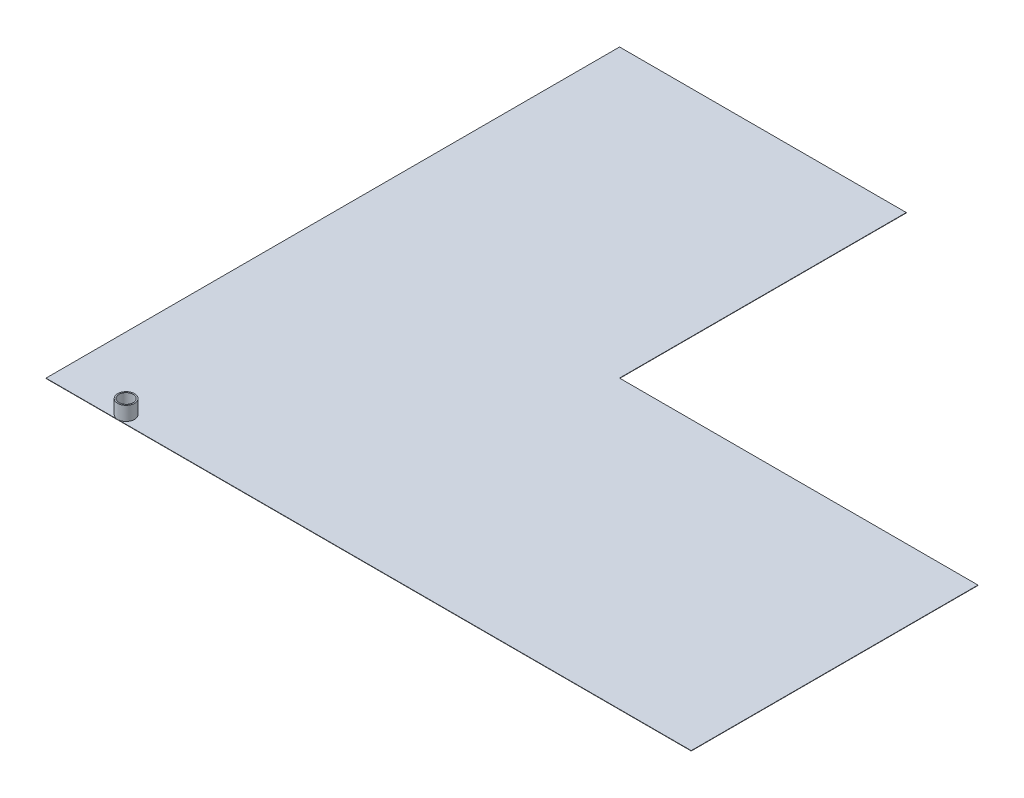
from build123d import *

# Parameters (mm, degrees)
BOSS_EXTRUDE1_DEPTH = 1
SKETCH2_R           = 20
CUT_EXTRUDE1_DEPTH  = 1205.159873107
BOSS_EXTRUDE2_START = 39
SKETCH3_R           = 23.5
SKETCH3_R_2         = 20
BOSS_EXTRUDE2_DEPTH = 39


with BuildPart() as part:
    # Sketch1 → Boss-Extrude1 (new body)
    with BuildSketch(Plane(origin=(0, 0, 0), x_dir=(1, 0, 0), z_dir=(0, 1, 0))):
        Polygon((-900, -800), (900, -800), (900, 0), (0, 0), (-100, 0), (-100, 800), (-900, 800), align=None)
    extrude(amount=BOSS_EXTRUDE1_DEPTH)

    # Sketch2 → Cut-Extrude1 (cut, through all)
    with BuildSketch(Plane(origin=(0, 1, 0), x_dir=(1, 0, 0), z_dir=(0, 1, 0))):
        with Locations(Location((-700, -776.5, 0), (0, 0, 270))):
            Circle(SKETCH2_R)
    extrude(amount=-CUT_EXTRUDE1_DEPTH, mode=Mode.SUBTRACT)

    # Sketch3 → Boss-Extrude2 (add)
    with BuildSketch(Plane(origin=(0, 1, 0), x_dir=(1, 0, 0), z_dir=(0, 1, 0)).offset(BOSS_EXTRUDE2_START)):
        with Locations(Location((-700, -776.5, 0), (0, 0, 270))):
            Circle(SKETCH3_R)
        with Locations(Location((-700, -776.5, 0), (0, 0, 270))):
            Circle(SKETCH3_R_2, mode=Mode.SUBTRACT)
    extrude(amount=-BOSS_EXTRUDE2_DEPTH)


solid = part.part
